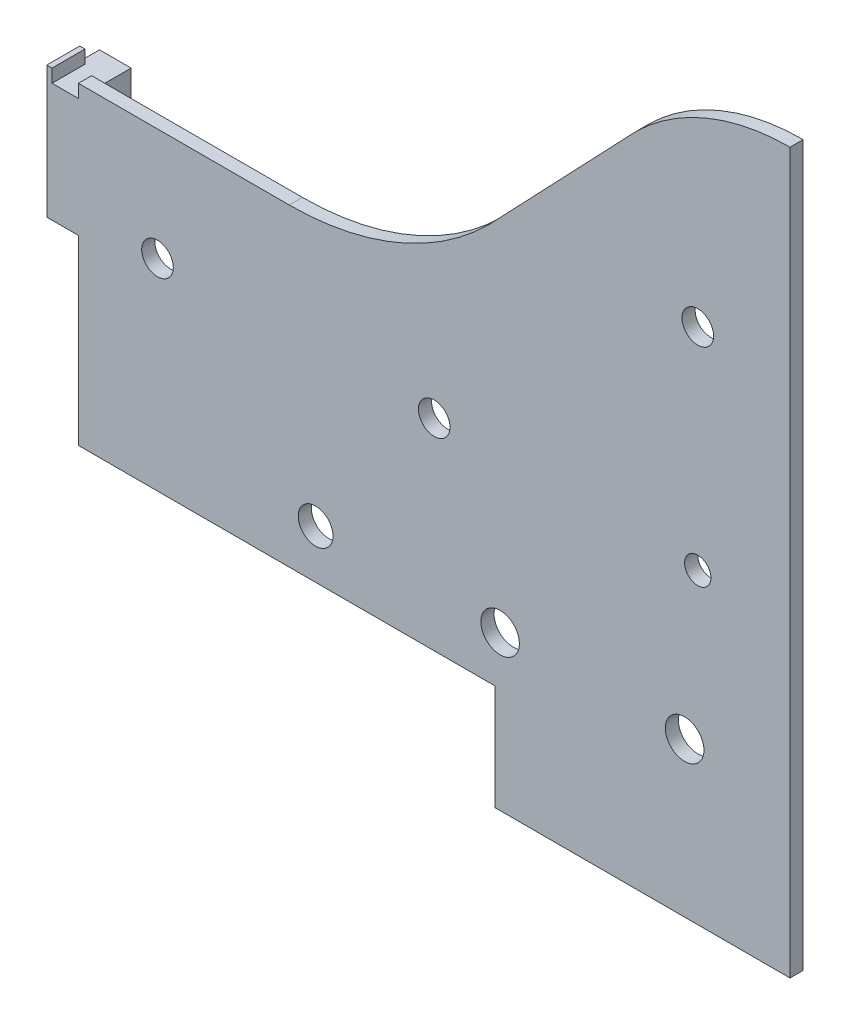
from build123d import *

# Parameters (mm, degrees)
EXTRUDE_3_DEPTH     = 5
SKETCH_2_W          = 12
SKETCH_2_H          = 20
EXTRUDE_4_DEPTH     = 50
CUT_EXTRUDE_1_DEPTH = 5
SKETCH_4_W          = 112
SKETCH_4_H          = 5
EXTRUDE_5_DEPTH     = 40
CUT_EXTRUDE_2_REACH = 1236.326
SKETCH_5_R          = 6
SKETCH_5_R_2        = 5
CUT_EXTRUDE_3_REACH = 1236.529
SKETCH_6_R          = 7.332886018
SKETCH_6_R_2        = 7.301331484
SKETCH_6_R_3        = 6.603217824


with BuildPart() as part:
    # 草图1 → 凸台-拉伸3 (new body)
    with BuildSketch(Plane.XY):
        with BuildLine():
            Line((-86.707495778, -188.910549606), (103.292504222, -188.910549606))
            Line((103.292504222, -188.910549606), (103.292504222, 44.089450394))
            ThreePointArc((103.292504222, 44.089450394), (71.593223998, 37.797700493), (44.699821924, 19.876333124))
            add(Edge.make_bspline(
                [(-10.94366291, -38.46742639), (16.878079507, -9.295546633), (44.699821924, 19.876333124)],
                knots=[-0.0017101, -0.0017101, -0.0017101, 0.998178008, 0.998178008, 0.998178008], degree=2))
            ThreePointArc((-10.94366291, -38.46742639), (-45.692777784, -61.737635508), (-86.707495778, -69.910549606))
            Line((-86.707495778, -69.910549606), (-166.707495778, -69.910549606))
            Line((-166.707495778, -69.910549606), (-166.707495778, -188.910549606))
            Line((-166.707495778, -188.910549606), (-86.707495778, -188.910549606))
        make_face()
    extrude(amount=EXTRUDE_3_DEPTH)

    # 草图2 → 凸台-拉伸4 (add)
    with BuildSketch(Plane(origin=(0, -69.910549606, 0), x_dir=(1, 0, 0), z_dir=(0, 1, 0))):
        with Locations((-172.707495778, 5)):
            Rectangle(SKETCH_2_W, SKETCH_2_H)
    extrude(amount=-EXTRUDE_4_DEPTH)

    # 草图3 → 切除-拉伸1 (cut)
    with BuildSketch(Plane(origin=(0, -69.910549606, 0), x_dir=(1, 0, 0), z_dir=(0, 1, 0))):
        Polygon((-166.707495778, 0), (-166.707495778, -5), (-176.720177385, -5), (-176.720177385, 7.5), (-178.707495778, 7.5), (-178.707495778, 15), (-166.707495778, 15), align=None)
    extrude(amount=-CUT_EXTRUDE_1_DEPTH, mode=Mode.SUBTRACT)

    # 草图4 → 凸台-拉伸5 (add)
    with BuildSketch(Plane.XZ.offset(188.910549606)):
        with Locations((47.292504222, 2.5)):
            Rectangle(SKETCH_4_W, SKETCH_4_H)
    extrude(amount=EXTRUDE_5_DEPTH)

    # 草图5 → 切除-拉伸2 (cut, up to next)
    with BuildSketch(Plane(origin=(703.41878585, 634.231928171, 5), x_dir=(0, 1, 0), z_dir=(0, 0, 1)), mode=Mode.PRIVATE) as cut_extrude_2_sk1:
        with Locations(Location((-666.704267343, 635.126281628, 0), (0, 0, 270))):
            Circle(SKETCH_5_R)
    cut_extrude_2_tool1 = extrude(cut_extrude_2_sk1.sketch, amount=-CUT_EXTRUDE_2_REACH, mode=Mode.PRIVATE) & part.part
    # 草图5 → 切除-拉伸2 (cut, up to next)
    with BuildSketch(Plane(origin=(703.41878585, 634.231928171, 5), x_dir=(0, 1, 0), z_dir=(0, 0, 1)), mode=Mode.PRIVATE) as cut_extrude_2_sk2:
        with Locations(Location((-746.704267343, 635.126281628, 0), (0, 0, 270))):
            Circle(SKETCH_5_R_2)
    cut_extrude_2_tool2 = extrude(cut_extrude_2_sk2.sketch, amount=-CUT_EXTRUDE_2_REACH, mode=Mode.PRIVATE) & part.part
    # 草图5 → 切除-拉伸2 (cut, up to next)
    with BuildSketch(Plane(origin=(703.41878585, 634.231928171, 5), x_dir=(0, 1, 0), z_dir=(0, 0, 1)), mode=Mode.PRIVATE) as cut_extrude_2_sk3:
        with Locations(Location((-746.704267343, 840.126281628, 0), (0, 0, 270))):
            Circle(SKETCH_5_R)
    cut_extrude_2_tool3 = extrude(cut_extrude_2_sk3.sketch, amount=-CUT_EXTRUDE_2_REACH, mode=Mode.PRIVATE) & part.part
    # 草图5 → 切除-拉伸2 (cut, up to next)
    with BuildSketch(Plane(origin=(703.41878585, 634.231928171, 5), x_dir=(0, 1, 0), z_dir=(0, 0, 1)), mode=Mode.PRIVATE) as cut_extrude_2_sk4:
        with Locations(Location((-746.704267343, 735.126281628, 0), (0, 0, 270))):
            Circle(SKETCH_5_R)
    cut_extrude_2_tool4 = extrude(cut_extrude_2_sk4.sketch, amount=-CUT_EXTRUDE_2_REACH, mode=Mode.PRIVATE) & part.part
    add(cut_extrude_2_tool1.solids().sort_by_distance((68.292504, -32.472339, 5))[0], mode=Mode.SUBTRACT)
    add(cut_extrude_2_tool2.solids().sort_by_distance((68.292504, -112.472339, 5))[0], mode=Mode.SUBTRACT)
    add(cut_extrude_2_tool3.solids().sort_by_distance((-136.707496, -112.472339, 5))[0], mode=Mode.SUBTRACT)
    add(cut_extrude_2_tool4.solids().sort_by_distance((-31.707496, -112.472339, 5))[0], mode=Mode.SUBTRACT)

    # 草图6 → 切除-拉伸3 (cut, up to next)
    with BuildSketch(Plane(origin=(703.41878585, 634.231928171, 15), x_dir=(0, 1, 0), z_dir=(0, 0, 1)), mode=Mode.PRIVATE) as cut_extrude_3_sk1:
        with Locations(Location((-804.642477777, 640.126281628, 0), (0, 0, 270))):
            Circle(SKETCH_6_R)
    cut_extrude_3_tool1 = extrude(cut_extrude_3_sk1.sketch, amount=-CUT_EXTRUDE_3_REACH, mode=Mode.PRIVATE) & part.part
    # 草图6 → 切除-拉伸3 (cut, up to next)
    with BuildSketch(Plane(origin=(703.41878585, 634.231928171, 15), x_dir=(0, 1, 0), z_dir=(0, 0, 1)), mode=Mode.PRIVATE) as cut_extrude_3_sk2:
        with Locations(Location((-804.642477777, 710.126281628, 0), (0, 0, 270))):
            Circle(SKETCH_6_R_2)
    cut_extrude_3_tool2 = extrude(cut_extrude_3_sk2.sketch, amount=-CUT_EXTRUDE_3_REACH, mode=Mode.PRIVATE) & part.part
    # 草图6 → 切除-拉伸3 (cut, up to next)
    with BuildSketch(Plane(origin=(703.41878585, 634.231928171, 15), x_dir=(0, 1, 0), z_dir=(0, 0, 1)), mode=Mode.PRIVATE) as cut_extrude_3_sk3:
        with Locations(Location((-804.642477777, 780.126281628, 0), (0, 0, 270))):
            Circle(SKETCH_6_R_3)
    cut_extrude_3_tool3 = extrude(cut_extrude_3_sk3.sketch, amount=-CUT_EXTRUDE_3_REACH, mode=Mode.PRIVATE) & part.part
    add(cut_extrude_3_tool1.solids().sort_by_distance((63.292504, -170.41055, 15))[0], mode=Mode.SUBTRACT)
    add(cut_extrude_3_tool2.solids().sort_by_distance((-6.707496, -170.41055, 15))[0], mode=Mode.SUBTRACT)
    add(cut_extrude_3_tool3.solids().sort_by_distance((-76.707496, -170.41055, 15))[0], mode=Mode.SUBTRACT)


solid = part.part
